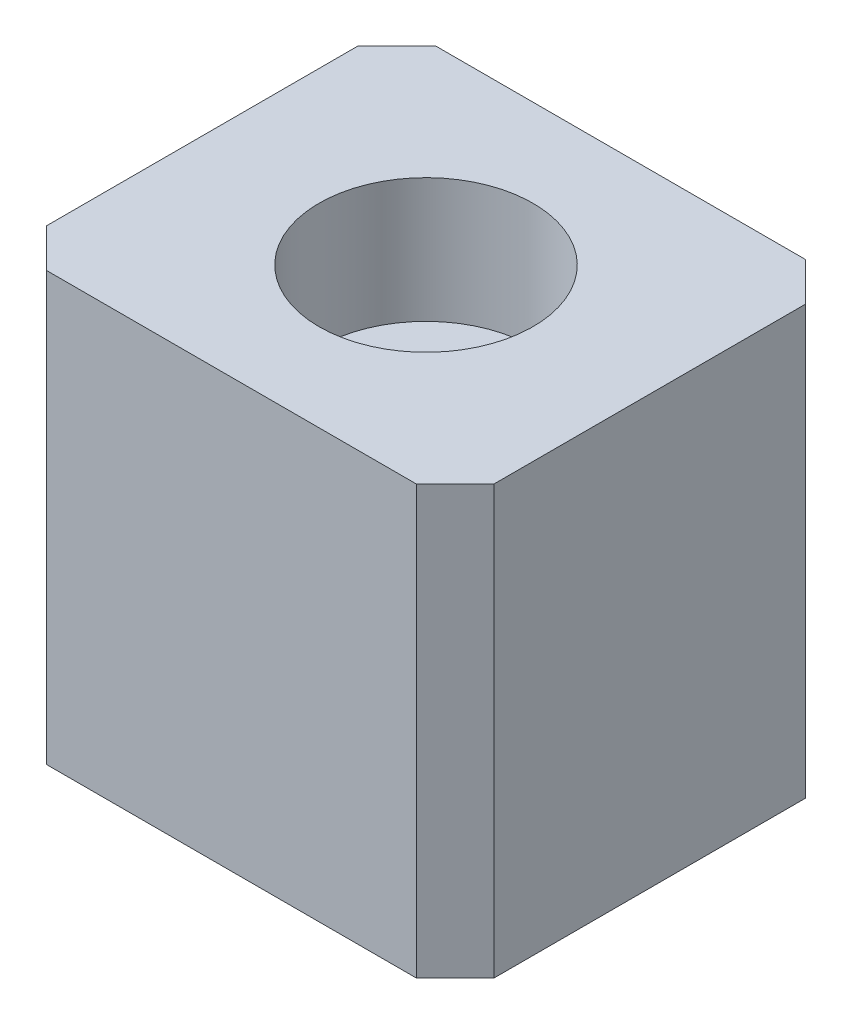
from build123d import *

# Parameters (mm, degrees)
SKETCH_1_W                   = 23
SKETCH_1_H                   = 20
EXTRUDE_1_DEPTH              = 11
HOLE_WIZARD_M6_1_D           = 6.6
HOLE_WIZARD_M6_1_CBORE_D     = 11
HOLE_WIZARD_M6_1_CBORE_DEPTH = 6.4
CHAMFER_1_SIZE               = 2


with BuildPart() as part:
    # 草图1 → 凸台-拉伸1 (new, symmetric)
    with BuildSketch(Plane(origin=(0, 0, 0), x_dir=(1, 0, 0), z_dir=(0, 1, 0))):
        Rectangle(SKETCH_1_W, SKETCH_1_H)
    extrude(amount=EXTRUDE_1_DEPTH, both=True)

    # M6 六角凹头螺钉的柱形沉头孔1 (through all)
    with Locations(Plane(origin=(0, 11, 0), x_dir=(1, 0, 0), z_dir=(0, 1, 0))):
        with Locations((0, 0)):
            CounterBoreHole(HOLE_WIZARD_M6_1_D / 2, HOLE_WIZARD_M6_1_CBORE_D / 2, HOLE_WIZARD_M6_1_CBORE_DEPTH)

    # 倒角1
    chamfer_1_edges = [part.edges().sort_by_distance(p)[0] for p in [
        (-11.5, 0, -10),
        (11.5, 0, -10),
        (11.5, 0, 10),
        (-11.5, 0, 10),
    ]]
    chamfer(chamfer_1_edges, length=CHAMFER_1_SIZE)


solid = part.part
